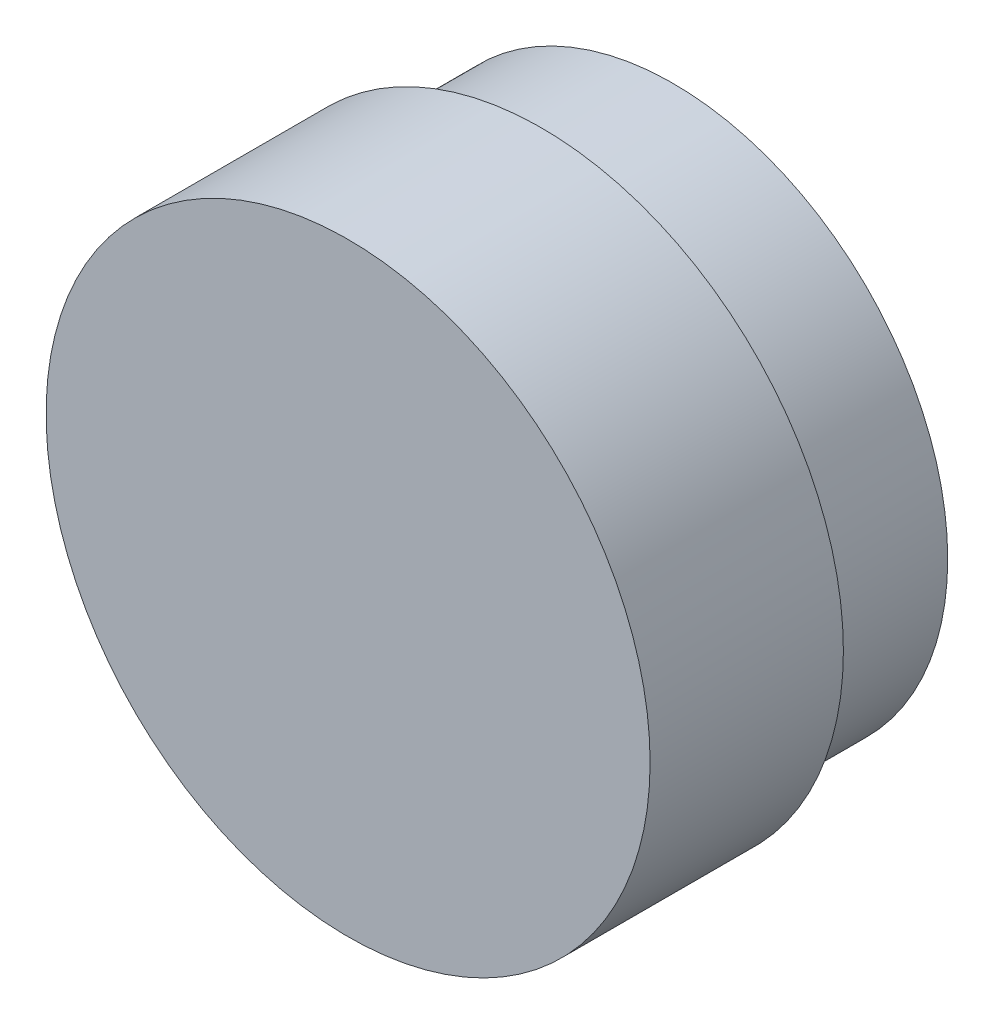
from build123d import *

# Parameters (mm, degrees)
SKETCH1_R           = 25
BOSS_EXTRUDE1_DEPTH = 12
SKETCH2_R           = 27.5
BOSS_EXTRUDE2_DEPTH = 17.6


with BuildPart() as part:
    # Sketch1 → Boss-Extrude1 (new body)
    with BuildSketch(Plane.XY):
        Circle(SKETCH1_R)
    extrude(amount=BOSS_EXTRUDE1_DEPTH)

    # Sketch2 → Boss-Extrude2 (add)
    with BuildSketch(Plane.XY.offset(12)):
        Circle(SKETCH2_R)
    extrude(amount=BOSS_EXTRUDE2_DEPTH)


solid = part.part
